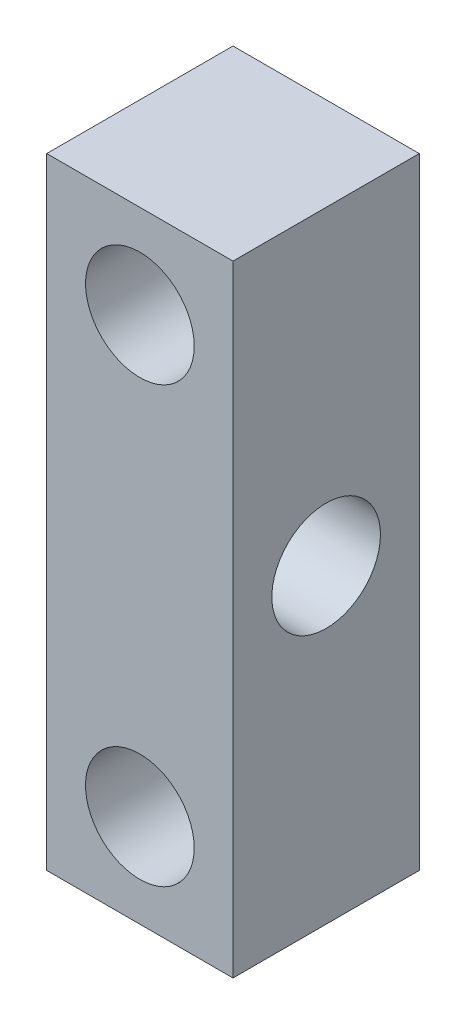
SolidWorks part; units mm, degrees
ref_plane "前视基准面" through (0, 0, 0) normal (0, 0, 1) x (1, 0, 0)
ref_plane "上视基准面" through (0, 0, 0) normal (0, 1, 0) x (1, 0, 0)
ref_plane "右视基准面" through (0, 0, 0) normal (1, 0, 0) x (0, 0, -1)
sketch "草图1" plane through (0, 0, 0) normal (0, 0, 1) x (1, 0, 0)
  line L1 (-6, -20) -> (6, -20)
  line L2 (-6, -20) -> (-6, 20)
  line L3 (-6, 20) -> (6, 20)
  line L4 (6, -20) -> (6, 20)
  line L5 (-6, -20) -> (6, 20) construction
  line L6 (-6, 20) -> (6, -20) construction
  circle A0 centre (0, 14) radius 3.5
  circle A1 centre (0, -14) radius 3.5
  point P0 (0, 0)
  dimension "D3" = 7
  dimension "D1" = 12
  dimension "D2" = 40
  dimension "D4" = 6
  dimension "D5" = 6
extrude "凸台-拉伸1" add sketch "草图1" along normal mid plane 12
sketch "草图2" plane through (6, 0, 0) normal (1, 0, 0) x (0, 0, -1)
  circle A0 centre (0, 0) radius 3.5
  dimension "D1" = 7
extrude "切除-拉伸1" cut sketch "草图2" against normal up to next
